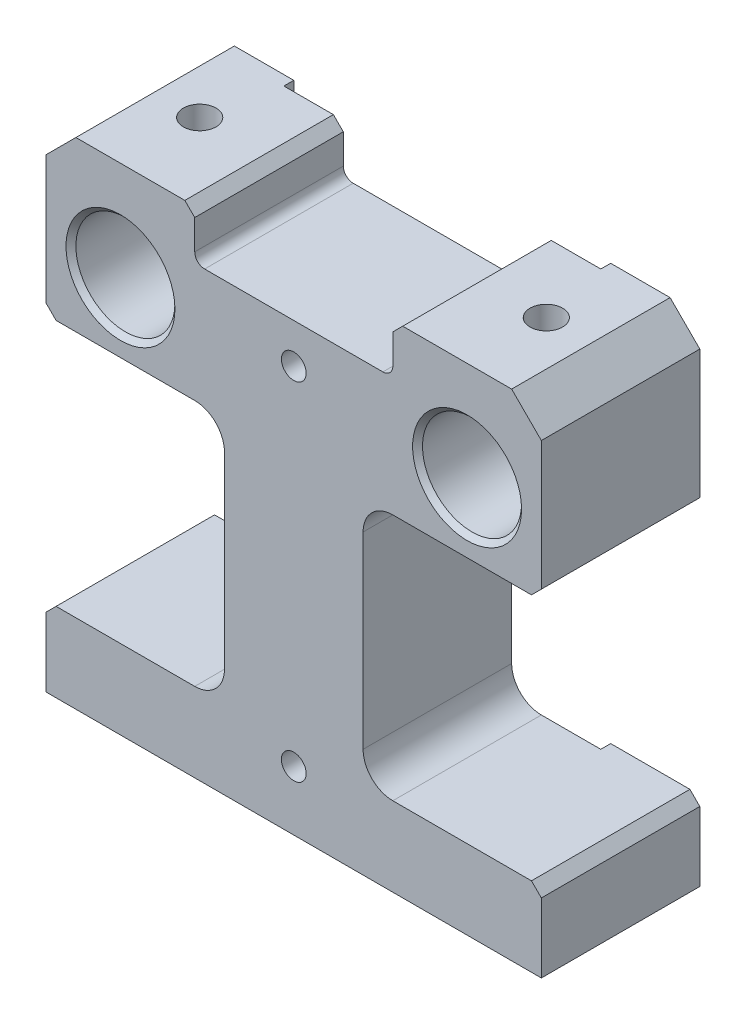
SolidWorks part; units mm, degrees
material "S45C"
ref_plane "Front Plane" through (0, 0, 0) normal (0, 0, 1) x (1, 0, 0)
ref_plane "Top Plane" through (0, 0, 0) normal (0, 1, 0) x (1, 0, 0)
ref_plane "Right Plane" through (0, 0, 0) normal (1, 0, 0) x (0, 0, -1)
sketch "Sketch1" plane through (0, 0, 0) normal (0, 0, 1) x (1, 0, 0)
  line L0 (0, 0) -> (0, -39.3421) construction
  line L1 (-55, -25) -> (55, -25)
  line L2 (-55, -25) -> (-55, 25)
  line L3 (-55, 25) -> (55, 25)
  line L4 (55, -25) -> (55, 25)
  line L5 (-55, -25) -> (55, 25) construction
  line L6 (-55, 25) -> (55, -25) construction
  line L7 (55, 25) -> (25, 25)
  line L8 (55, 25) -> (55, -10)
  line L9 (55, -10) -> (25, -10)
  line L10 (25, 25) -> (25, -10)
  line L11 (-55, 25) -> (-25, 25)
  line L12 (-55, 25) -> (-55, -10)
  line L13 (-55, -10) -> (-25, -10)
  line L14 (-25, 25) -> (-25, -10)
  line L15 (25, -10) -> (25, -25)
  line L16 (-25, -10) -> (-25, -25)
  point P0 (0, 0)
  dimension "D1" = 15
  dimension "D2" = 50
  dimension "D3" = 50
  dimension "D4" = 110
extrude "Boss-Extrude1" add sketch "Sketch1" along normal mid plane 16 contours L3 L14 L13 L2 L1 L4 L9 L10
sketch "Sketch6" plane through (0, 0, 8) normal (0, 0, 1) x (1, 0, 0)
  line L0 (0, 0) -> (0, 39.092) construction
  line L1 (-25, -25) -> (25, -25) construction
  line L3 (7, 8) -> (25, 8)
  line L4 (7, 8) -> (7, -17)
  line L5 (7, -17) -> (25, -17)
  line L6 (25, 8) -> (25, -17)
  line L7 (-25, 25) -> (25, 25) construction
  line L8 (25, 25) -> (25, -25) construction
  line L9 (-25, 25) -> (-25, -25) construction
  line L10 (-25, 8) -> (-7, 8)
  line L11 (-25, 8) -> (-25, -17)
  line L12 (-25, -17) -> (-7, -17)
  line L13 (-7, 8) -> (-7, -17)
  circle A0 centre (-17.5, 15) radius 5
  circle A1 centre (17.5, 15) radius 5
  dimension "D1" = 10
  dimension "D2" = 35
  dimension "D3" = 40
  dimension "D4" = 18
  dimension "D5" = 25
  dimension "D6" = 17
extrude "Cut-Extrude1" cut sketch "Sketch6" against normal through all
hole_wizard "M4 Tapped Hole1" positions "Sketch8" profile "Sketch7" tap size "M4" standard "GB"
sketch "Sketch8" plane through (0, 25, 0) normal (0, 1, 0) x (1, 0, 0)
  line L0 (-17.5, 8) -> (-17.5, -8) construction
  line L4 (17.5, 8) -> (17.5, -8) construction
  line L6 (-25, 8) -> (25, 8) construction
  line L7 (22.5, 8) -> (12.5, 8) construction
  line L8 (-12.5, 8) -> (-22.5, 8) construction
  line L9 (-25, -8) -> (25, -8) construction
  point P0 (-17.5, 0)
  point P2 (17.5, 0)
sketch "Sketch7" plane through (-17.5, 25, 0) normal (1, 0, 0) x (0, 0, 1)
  line L0 (0, 0) -> (0, 5)
  line L1 (0, 5) -> (1.65, 5)
  line L2 (1.65, 5) -> (1.65, 0)
  line L5 (1.65, 0) -> (0, 0)
  line L11 (0, -6.35) -> (0, 107.95) construction
  dimension "通孔螺纹孔钻头直径" = 3.3
  dimension "通孔螺纹孔钻头深度" = 5
cosmetic thread "Cosmetic Thread 1" parameters "D2"=4
cosmetic thread "Cosmetic Thread 4" parameters "D2"=4
hole_wizard "M3 Tapped Hole1" positions "Sketch10" profile "Sketch9" tap size "M3" standard "GB" end condition up to next
sketch "Sketch10" plane through (0, 0, 8) normal (0, 0, 1) x (1, 0, 0)
  line L0 (-25, -25) -> (25, -25) construction
  point P0 (0, -19)
  point P2 (0, 16)
  dimension "D1" = 6
  dimension "D2" = 35
sketch "Sketch9" plane through (0, -19, 8) normal (1, 0, 0) x (0, -1, 0)
  line L0 (0, 0) -> (0, 16)
  line L1 (0, 16) -> (1.25, 16)
  line L2 (1.25, 16) -> (1.25, 0)
  line L5 (1.25, 0) -> (0, 0)
  line L11 (0, -6.35) -> (0, 107.95) construction
  dimension "通孔螺纹孔钻头直径" = 2.5
  dimension "通孔螺纹孔钻头深度" = 16
cosmetic thread "Cosmetic Thread 5" parameters "D2"=3
cosmetic thread "Cosmetic Thread 6" parameters "D2"=3
sketch "Sketch13" plane through (0, 0, -8) normal (0, 0, 1) x (1, 0, 0)
  line L0 (-25, -25) -> (25, -25) construction
  line L1 (-16, -25) -> (16, -25)
  line L2 (-16, -25) -> (-16, 25)
  line L3 (-16, 25) -> (16, 25)
  line L4 (16, -25) -> (16, 25)
  line L5 (-25, 25) -> (25, 25) construction
  line L6 (0, 0) -> (0, -14.5924) construction
  dimension "D1" = 32
extrude "Cut-Extrude2" cut sketch "Sketch13" along normal blind 1
sketch "Sketch14" plane through (0, 0, 8) normal (0, 0, 1) x (1, 0, 0)
  line L0 (-25, 25) -> (25, 25) construction
  line L1 (-10, 25) -> (10, 25)
  line L2 (-10, 25) -> (-10, 20)
  line L3 (-10, 20) -> (10, 20)
  line L4 (10, 25) -> (10, 20)
  line L5 (0, 0) -> (0, 11.4869) construction
  dimension "D1" = 20
  dimension "D2" = 5
extrude "Cut-Extrude3" cut sketch "Sketch14" against normal through all
chamfer "Chamfer1" distance 3 angle 45 2 edges at (25, 25, 0) (-25, 25, 0)
fillet "Fillet1" radius 3 4 edges at (7, -17, 0.5) (7, 8, 0.5) (-7, -17, 0.5) (-7, 8, 0.5)
chamfer "Chamfer3" distance 1 angle 45 6 edges at (25, -17, 0) (25, 8, 0) (-25, 8, 0) (-25, -17, 0) (10, 25, 0.5) (-10, 25, 0.5)
chamfer "Chamfer4" distance 0.5 angle 45 4 edges at (22.5, 15, -8) (-22.5, 15, -8) (22.5, 15, 8) (-12.5, 15, 8)
fillet "Fillet2" radius 1 2 edges at (10, 20, 0.5) (-10, 20, 0.5)
